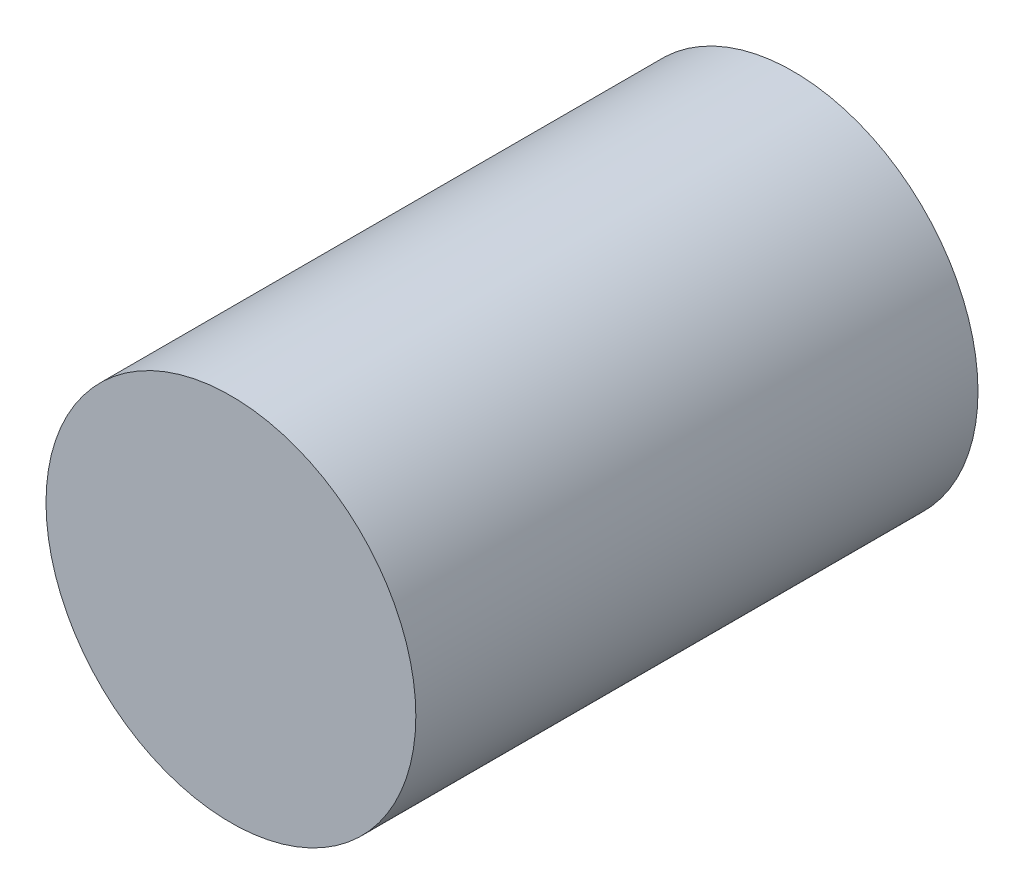
from build123d import *

# Parameters (mm, degrees)
BOSS_EXTRUDE1_DEPTH      = 5
BOSS_EXTRUDE1_DEPTH_BACK = 33
SKETCH1_R                = 12.5


with BuildPart() as part:
    # Sketch1 → Boss-Extrude1 (new, two sides: drawn at the far end of the back side and taken through both)
    with BuildSketch(Plane.XY.offset(-BOSS_EXTRUDE1_DEPTH_BACK)):
        with Locations((432.939239469, 69.231267182)):
            Circle(SKETCH1_R)
    extrude(amount=BOSS_EXTRUDE1_DEPTH + BOSS_EXTRUDE1_DEPTH_BACK)


solid = part.part
